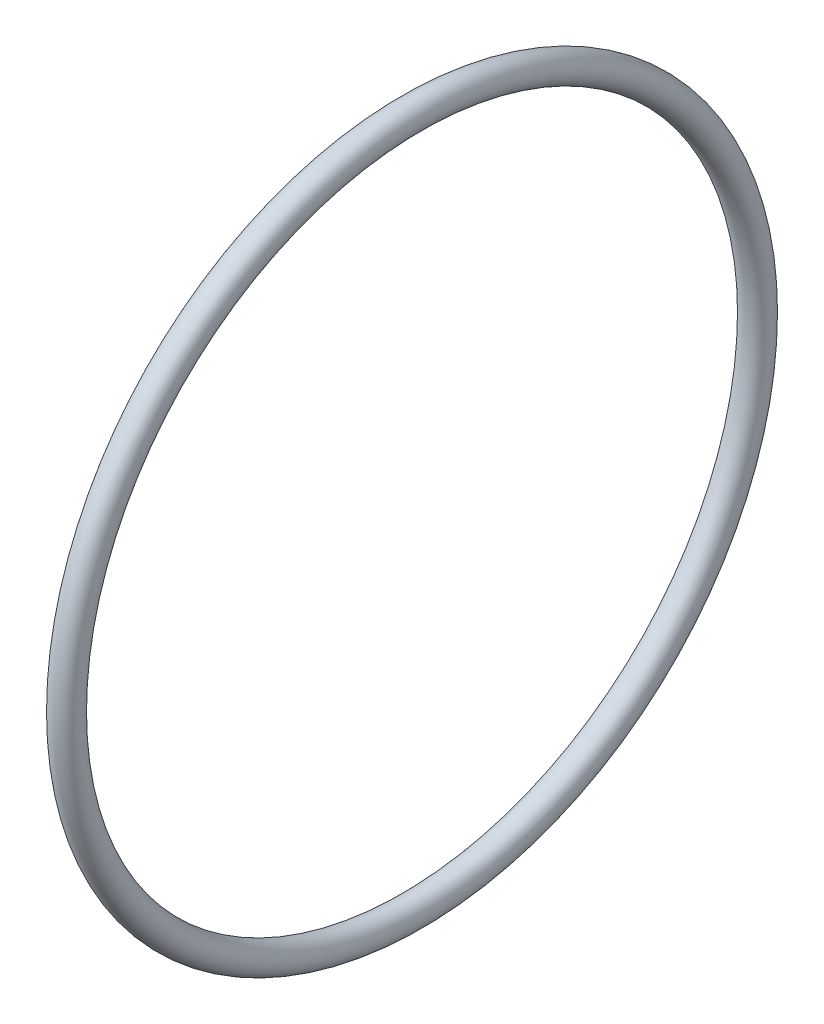
from build123d import *

# Parameters (mm, degrees)
SKETCH1_R = 1.325


with BuildPart() as part:
    # Sketch1 → Revolve1 (revolve)
    with BuildSketch(Plane.XY, mode=Mode.PRIVATE) as revolve1_sk:
        with Locations((5, 32.35)):
            Circle(SKETCH1_R)
    revolve(revolve1_sk.sketch.rotate(Axis((0, 0, 0), (1, 0, 0)), 90), axis=Axis((0, 0, 0), (1, 0, 0)))


solid = part.part
